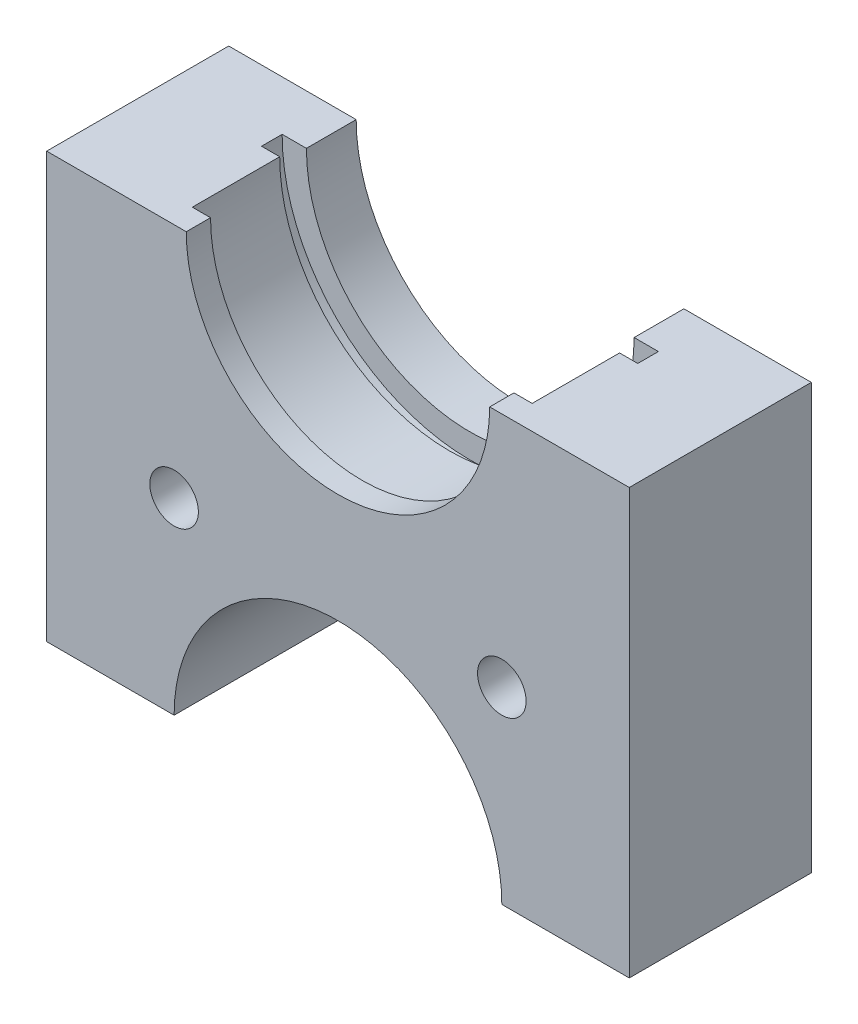
SolidWorks part; units mm, degrees
ref_plane "前视基准面" through (0, 0, 0) normal (0, 0, 1) x (1, 0, 0)
ref_plane "上视基准面" through (0, 0, 0) normal (0, 1, 0) x (1, 0, 0)
ref_plane "右视基准面" through (0, 0, 0) normal (1, 0, 0) x (0, 0, -1)
sketch "草图1" plane through (0, 0, 0) normal (0, 0, 1) x (1, 0, 0)
  line L1 (-240, 175) -> (240, 175)
  line L2 (-240, 175) -> (-240, -175)
  line L3 (-240, -175) -> (240, -175)
  line L4 (240, 175) -> (240, -175)
  line L5 (-240, 175) -> (240, -175) construction
  line L6 (-240, -175) -> (240, 175) construction
  point P0 (0, 0)
  point P5 (0, 0)
  dimension "D1" = 480
  dimension "D2" = 350
extrude "凸台-拉伸1" add sketch "草图1" along normal blind 150
sketch "草图2" plane through (0, 0, 150) normal (0, 0, 1) x (1, 0, 0)
  line L0 (0, 0) -> (0, -175) construction
  line L1 (-240, -175) -> (240, -175) construction
  circle A0 centre (-135, -20) radius 20
  circle A1 centre (135, -20) radius 20
  dimension "D1" = 40
  dimension "D2" = 135
  dimension "D3" = 155
extrude "切除-拉伸1" cut sketch "草图2" against normal through all both and the other way through all
sketch "草图3" plane through (0, 0, 150) normal (0, 0, 1) x (1, 0, 0)
  line L0 (-240, -175) -> (240, -175) construction
  line L1 (0, 0) -> (240, 0) construction
  line L2 (240, -175) -> (240, 175) construction
  line L3 (240, 175) -> (-240, 175) construction
  circle A0 centre (0, -175) radius 135
  circle A1 centre (0, 175) radius 125
  dimension "D1" = 270
  dimension "D2" = 250
extrude "切除-拉伸2" cut sketch "草图3" against normal through all both and the other way through all
sketch "草图5" plane through (0, 175, 0) normal (0, 1, 0) x (1, 0, 0)
  line L0 (0, -150) -> (0, -130) construction
  line L1 (-125, -150) -> (125, -150) construction
  line L2 (0, -130) -> (-140, -130)
  line L3 (-140, -130) -> (-140, -58)
  line L4 (-140, -58) -> (-155, -58)
  line L5 (-155, -58) -> (-155, -41)
  line L6 (-155, -41) -> (-135, -41)
  line L7 (0, -41) -> (0, -130)
  line L8 (-135, -41) -> (-135, 0)
  line L9 (-135, 0) -> (0, 0)
  line L10 (125, 0) -> (-125, 0) construction
  line L11 (0, 0) -> (0, -41)
  dimension "D1" = 20
  dimension "D2" = 72
  dimension "D3" = 140
  dimension "D4" = 155
  dimension "D5" = 89
revolve "切除-旋转1" cut sketch "草图5" angle 360 about L0
